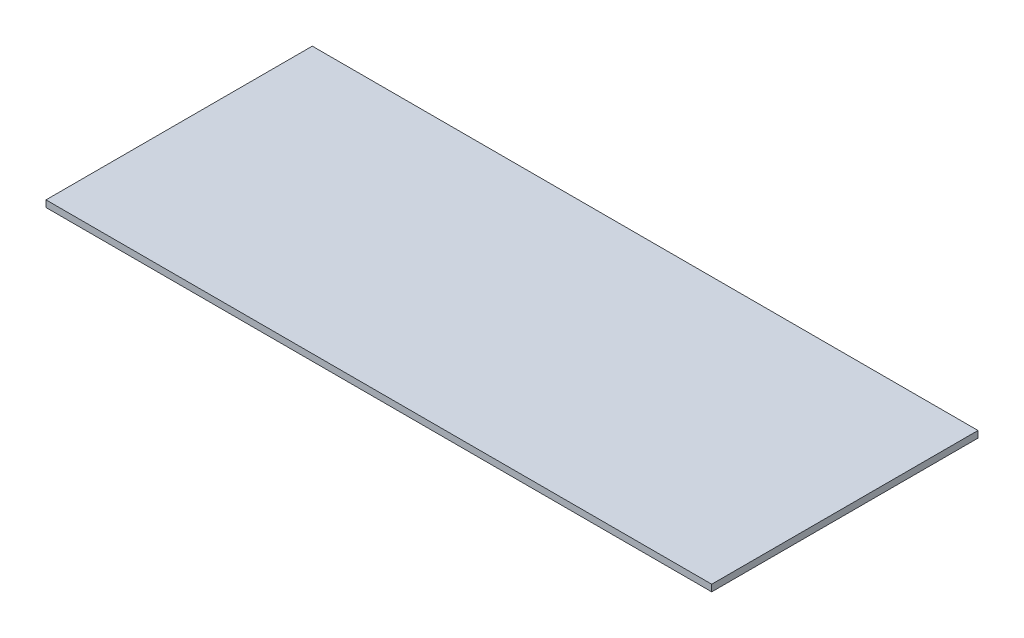
from build123d import *

# Parameters (mm, degrees)
SKETCH_1_W      = 100
SKETCH_1_H      = 40
EXTRUDE_1_DEPTH = 1


with BuildPart() as part:
    # 草图1 → 凸台-拉伸1 (new body)
    with BuildSketch(Plane(origin=(0, 0, 0), x_dir=(1, 0, 0), z_dir=(0, 1, 0))):
        Rectangle(SKETCH_1_W, SKETCH_1_H)
    extrude(amount=EXTRUDE_1_DEPTH)


solid = part.part
